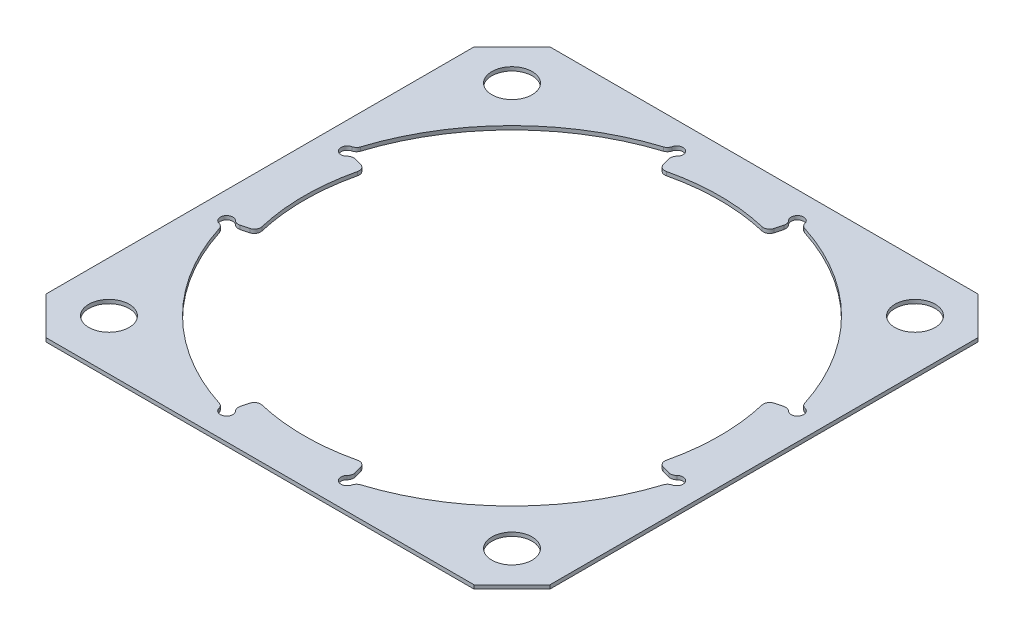
from build123d import *

# Parameters (mm, degrees)
BOSS_EXTRUDE1_DEPTH = 0.3
CUT_EXTRUDE1_DEPTH  = 0.4
SKETCH3_R           = 0.5
CUT_EXTRUDE2_DEPTH  = 0.4
FILLET1_R           = 0.5
SKETCH4_R           = 1.6
CUT_EXTRUDE3_DEPTH  = 0.4


with BuildPart() as part:
    # Sketch1 → Boss-Extrude1 (new body)
    with BuildSketch(Plane(origin=(0, 0, 0), x_dir=(1, 0, 0), z_dir=(0, 1, 0))):
        Polygon((-20, 17), (-17, 20), (17, 20), (20, 17), (20, -17), (17, -20), (-17, -20), (-20, -17), align=None)
    extrude(amount=BOSS_EXTRUDE1_DEPTH)

    # Sketch2 → Cut-Extrude1 (cut)
    with BuildSketch(Plane(origin=(0, 0.3, 0), x_dir=(1, 0, 0), z_dir=(0, 1, 0))):
        with BuildLine():
            Line((-17.386664873, 4.658742812), (-15.937776134, 4.270514244))
            ThreePointArc((-15.937776134, 4.270514244), (-16.5, 0), (-15.937776134, -4.270514244))
            Line((-15.937776134, -4.270514244), (-17.386664873, -4.658742812))
            ThreePointArc((-17.386664873, -4.658742812), (-17.616707665, -4.356838745), (-17.992498966, -4.303484744))
            ThreePointArc((-17.992498966, -4.303484744), (-13.081475452, -13.081475452), (-4.303484744, -17.992498966))
            ThreePointArc((-4.303484744, -17.992498966), (-4.356838745, -17.616707665), (-4.658742812, -17.386664873))
            Line((-4.658742812, -17.386664873), (-4.270514244, -15.937776134))
            ThreePointArc((-4.270514244, -15.937776134), (0, -16.5), (4.270514244, -15.937776134))
            Line((4.270514244, -15.937776134), (4.658742812, -17.386664873))
            ThreePointArc((4.658742812, -17.386664873), (4.356838745, -17.616707665), (4.303484744, -17.992498966))
            ThreePointArc((4.303484744, -17.992498966), (13.081475452, -13.081475452), (17.992498966, -4.303484744))
            ThreePointArc((17.992498966, -4.303484744), (17.616707665, -4.356838745), (17.386664873, -4.658742812))
            Line((17.386664873, -4.658742812), (15.937776134, -4.270514244))
            ThreePointArc((15.937776134, -4.270514244), (16.5, 0), (15.937776134, 4.270514244))
            Line((15.937776134, 4.270514244), (17.386664873, 4.658742812))
            ThreePointArc((17.386664873, 4.658742812), (17.616707665, 4.356838745), (17.992498966, 4.303484744))
            ThreePointArc((17.992498966, 4.303484744), (13.081475452, 13.081475452), (4.303484744, 17.992498966))
            ThreePointArc((4.303484744, 17.992498966), (4.356838745, 17.616707665), (4.658742812, 17.386664873))
            Line((4.658742812, 17.386664873), (4.270514244, 15.937776134))
            ThreePointArc((4.270514244, 15.937776134), (0, 16.5), (-4.270514244, 15.937776134))
            Line((-4.270514244, 15.937776134), (-4.658742812, 17.386664873))
            ThreePointArc((-4.658742812, 17.386664873), (-4.356838745, 17.616707665), (-4.303484744, 17.992498966))
            ThreePointArc((-4.303484744, 17.992498966), (-13.081475452, 13.081475452), (-17.992498966, 4.303484744))
            ThreePointArc((-17.992498966, 4.303484744), (-17.616707665, 4.356838745), (-17.386664873, 4.658742812))
        make_face()
    extrude(amount=-CUT_EXTRUDE1_DEPTH, mode=Mode.SUBTRACT)

    # Sketch3 → Cut-Extrude2 (cut)
    with BuildSketch(Plane(origin=(0, 0.3, 0), x_dir=(1, 0, 0), z_dir=(0, 1, 0))):
        with Locations((-17.869627786, 4.788152334)):
            Circle(SKETCH3_R)
        with Locations((-17.869627786, -4.788152334)):
            Circle(SKETCH3_R)
        with Locations((4.788152334, 17.869627786)):
            Circle(SKETCH3_R)
        with Locations((-4.788152334, 17.869627786)):
            Circle(SKETCH3_R)
        with Locations((17.869627786, -4.788152334)):
            Circle(SKETCH3_R)
        with Locations((17.869627786, 4.788152334)):
            Circle(SKETCH3_R)
        with Locations((-4.788152334, -17.869627786)):
            Circle(SKETCH3_R)
        with Locations((4.788152334, -17.869627786)):
            Circle(SKETCH3_R)
    extrude(amount=-CUT_EXTRUDE2_DEPTH, mode=Mode.SUBTRACT)

    # Fillet1
    fillet1_edges = [part.edges().sort_by_distance(p)[0] for p in [
        (-5.26932237, 0.15, 17.733703555),
        (17.733703555, 0.15, 5.26932237),
        (5.26932237, 0.15, -17.733703555),
        (-17.733703555, 0.15, -5.26932237),
        (-5.26932237, 0.15, -17.733703555),
        (-17.733703555, 0.15, 5.26932237),
        (5.26932237, 0.15, 17.733703555),
        (17.733703555, 0.15, -5.26932237),
        (-15.937776134, 0.15, 4.270514244),
        (-15.937776134, 0.15, -4.270514244),
        (-17.386664873, 0.15, -4.658742812),
        (-4.658742812, 0.15, -17.386664873),
        (-4.270514244, 0.15, -15.937776134),
        (4.270514244, 0.15, -15.937776134),
        (4.658742812, 0.15, -17.386664873),
        (17.386664873, 0.15, -4.658742812),
        (15.937776134, 0.15, -4.270514244),
        (15.937776134, 0.15, 4.270514244),
        (17.386664873, 0.15, 4.658742812),
        (4.658742812, 0.15, 17.386664873),
        (4.270514244, 0.15, 15.937776134),
        (-4.270514244, 0.15, 15.937776134),
        (-4.658742812, 0.15, 17.386664873),
        (-17.386664873, 0.15, 4.658742812),
    ]]
    fillet(fillet1_edges, radius=FILLET1_R)

    # Sketch4 → Cut-Extrude3 (cut)
    with BuildSketch(Plane(origin=(0, 0.3, 0), x_dir=(1, 0, 0), z_dir=(0, 1, 0))):
        with Locations(Location((-16, 16, 0), (0, 0, 270))):
            Circle(SKETCH4_R)
        with Locations(Location((16, 16, 0), (0, 0, 90))):
            Circle(SKETCH4_R)
        with Locations(Location((16, -16, 0), (0, 0, 270))):
            Circle(SKETCH4_R)
        with Locations(Location((-16, -16, 0), (0, 0, 90))):
            Circle(SKETCH4_R)
    extrude(amount=-CUT_EXTRUDE3_DEPTH, mode=Mode.SUBTRACT)


solid = part.part
